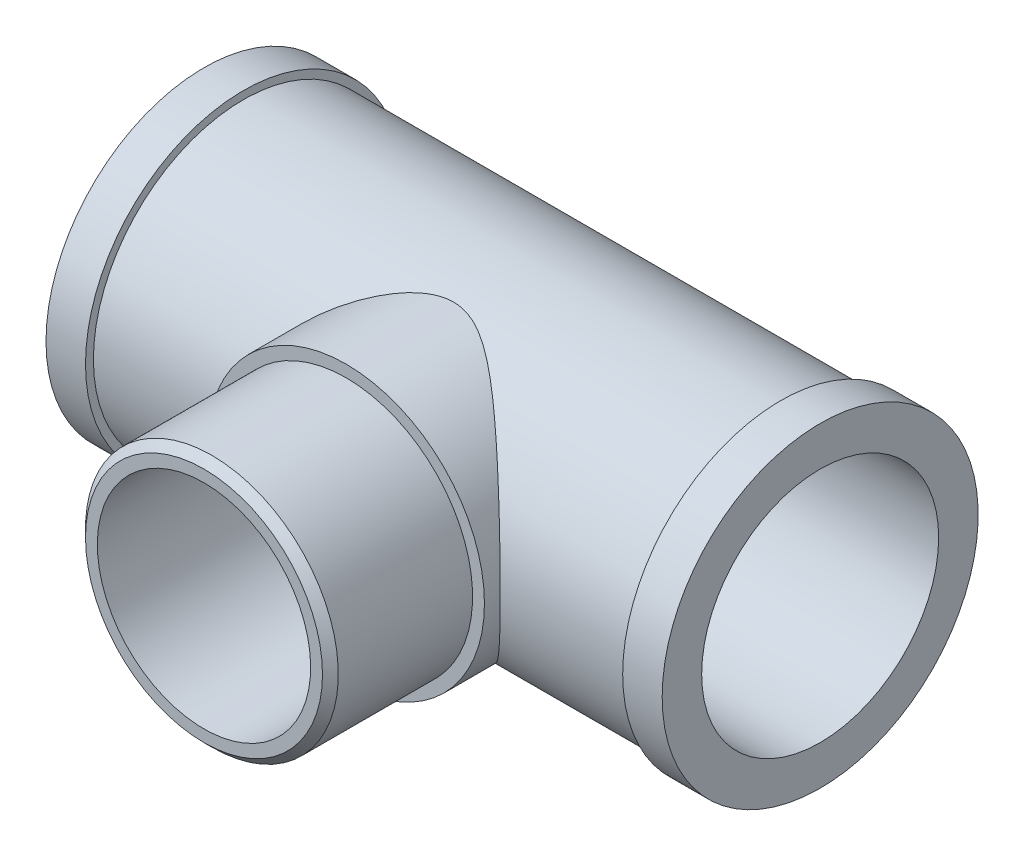
SolidWorks part; units mm, degrees
material "PP 共聚物"
ref_plane "Front Plane" through (0, 0, 0) normal (0, 0, 1) x (1, 0, 0)
ref_plane "Top Plane" through (0, 0, 0) normal (0, 1, 0) x (1, 0, 0)
ref_plane "Right Plane" through (0, 0, 0) normal (1, 0, 0) x (0, 0, -1)
sketch "Sketch1" plane through (0, 0, 0) normal (0, 0, 1) x (1, 0, 0)
  line L0 (5, 19) -> (5, 20)
  line L1 (5, 20) -> (0, 20)
  line L2 (0, 20) -> (0, 15)
  line L3 (0, 15) -> (0, 0) construction
  line L4 (78, 20) -> (73, 20)
  line L5 (73, 20) -> (73, 19)
  line L6 (73, 19) -> (5, 19)
  line L8 (78, 20) -> (78, 15)
  line L9 (78, 15) -> (0, 15)
  line L10 (0, 0) -> (59.4457, 0) construction
  dimension "D4" = 5
  dimension "D9" = 38
  dimension "D1" = 78
  dimension "D2" = 30
  dimension "D7" = 40
revolve "Revolve1" add sketch "Sketch1" angle 360 about L10
ref_plane "Plane1" through (39, 0, 0) normal (1, 0, 0) x (0, 0, -1)
sketch "Sketch3" plane through (39, 0, 0) normal (1, 0, 0) x (0, 0, -1)
  line L0 (0, 0) -> (-65.1795, 0) construction
  line L1 (-20, 0) -> (-20, -32.7671) construction
  line L3 (-39, -13.5) -> (-39, -16)
  line L4 (-39, -16) -> (-21, -16)
  line L5 (-21, -16) -> (-21, -17.5)
  line L6 (-21, -17.5) -> (-6.5383, -17.5)
  line L10 (-39, -13.5) -> (-6.5383, -13.5)
  line L11 (-6.5383, -17.5) -> (-6.5383, -13.5)
  circle A1 centre (0, 0) radius 20 construction
  circle A2 centre (0, 0) radius 15 construction
  dimension "D1" = 27
  dimension "D2" = 32
  dimension "D3" = 35
  dimension "D4" = 1
  dimension "D5" = 19
revolve "Revolve2" add sketch "Sketch3" angle 360 about L0
sketch "Sketch4" plane through (0, 0, 0) normal (-1, 0, 0) x (0, 0, 1)
  circle A0 centre (0, 0) radius 15 construction
  circle A1 centre (0, 0) radius 15
extrude "Cut-Extrude1" cut sketch "Sketch4" against normal through all
sketch "Sketch5" plane through (0, 0, 39) normal (0, 0, 1) x (1, 0, 0)
  circle A0 centre (39, 0) radius 13.5 construction
  circle A1 centre (39, 0) radius 13.5
extrude "Cut-Extrude2" cut sketch "Sketch5" against normal up to surface (24 mm away)
chamfer "Chamfer1" distance 1 angle 45 1 edges at (39, 16, 39)
